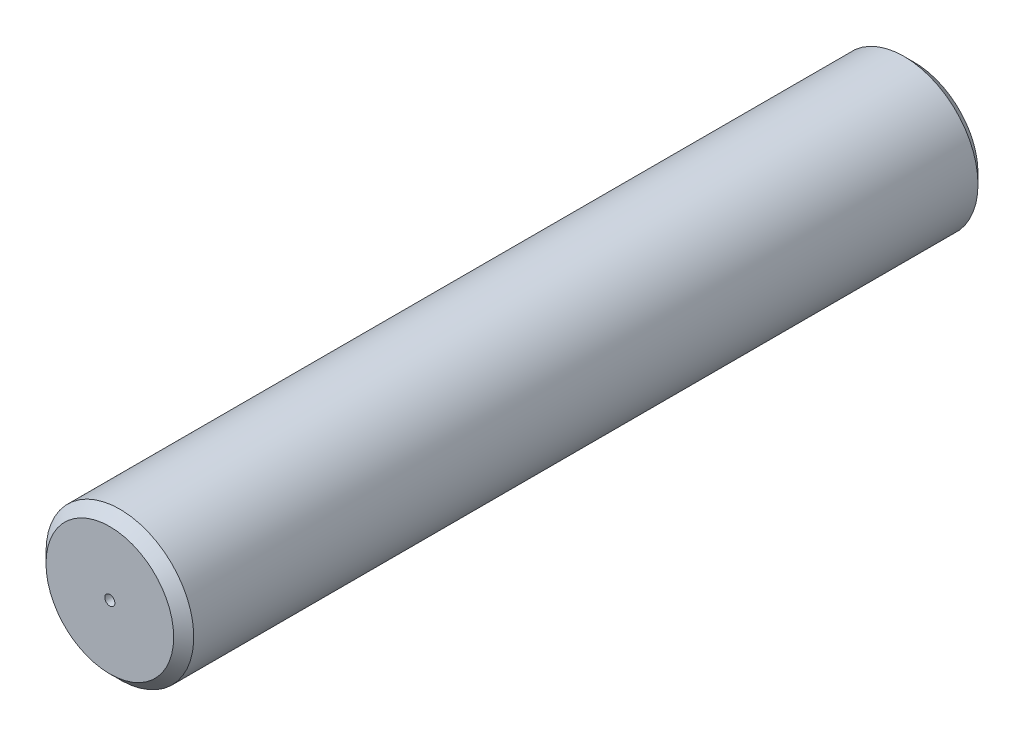
from build123d import *

# Parameters (mm, degrees)
SKETCH1_R               = 3.674588618
BOSS_EXTRUDE1_DEPTH     = 20
CHAMFER2_SIZE           = 0.5
SKETCH2_R               = 0.25
CUT_EXTRUDE1_DEPTH      = 1
CUT_EXTRUDE1_DRAFT      = -3
MIRROR1_COPY_1_SKETCH_R = 0.25
MIRROR1_COPY_1_DEPTH    = 1
MIRROR1_COPY_1_DRAFT    = -3


with BuildPart() as part:
    # Sketch1 → Boss-Extrude1 (new, symmetric)
    with BuildSketch(Plane.XY):
        with Locations(Location((-27.065651732, 0, 0), (0, 0, 180))):
            Circle(SKETCH1_R)
    extrude(amount=BOSS_EXTRUDE1_DEPTH, both=True)

    # Chamfer2
    chamfer2_edges = [part.edges().sort_by_distance(p)[0] for p in [
        (-23.391063114, 0, -20),
        (-23.391063114, 0, 20),
    ]]
    chamfer(chamfer2_edges, length=CHAMFER2_SIZE)


with BuildPart() as cut_extrude1_tool:
    # Sketch2 → Cut-Extrude1 (with draft: the straight prism first)
    with BuildSketch(Plane.XY.offset(20)):
        with Locations((-27.065651732, 0)):
            Circle(SKETCH2_R)
    extrude(amount=-CUT_EXTRUDE1_DEPTH)
    # Cut-Extrude1: the draft: its side faces are tilted about the plane it starts from
    cut_extrude1_sides = [cut_extrude1_tool.faces().sort_by_distance(p)[0] for p in [
        (-27.315651732, 0, 19.5),
    ]]
    draft(cut_extrude1_sides, Plane.XY.offset(20), CUT_EXTRUDE1_DRAFT)


with BuildPart() as part_1:
    add(part.part)

    # Cut-Extrude1: cut by cut_extrude1_tool
    add(cut_extrude1_tool.part, mode=Mode.SUBTRACT)


with BuildPart() as mirror1_copy_1_tool:
    # Mirror1 copy 1 sketch → Mirror1 copy 1 (with draft: the straight prism first)
    with BuildSketch(Plane(origin=(0, 0, -20), x_dir=(1, 0, 0), z_dir=(0, 0, -1))):
        with Locations((-27.065651732, 0)):
            Circle(MIRROR1_COPY_1_SKETCH_R)
    extrude(amount=-MIRROR1_COPY_1_DEPTH)
    # Mirror1 copy 1: the draft: its side faces are tilted about the plane it starts from
    mirror1_copy_1_sides = [mirror1_copy_1_tool.faces().sort_by_distance(p)[0] for p in [
        (-27.315651732, 0, -19.5),
    ]]
    draft(mirror1_copy_1_sides, Plane(origin=(0, 0, -20), x_dir=(1, 0, 0), z_dir=(0, 0, -1)), MIRROR1_COPY_1_DRAFT)


with BuildPart() as part_2:
    add(part_1.part)

    # Mirror1 copy 1: cut by mirror1_copy_1_tool
    add(mirror1_copy_1_tool.part, mode=Mode.SUBTRACT)


solid = part_2.part
